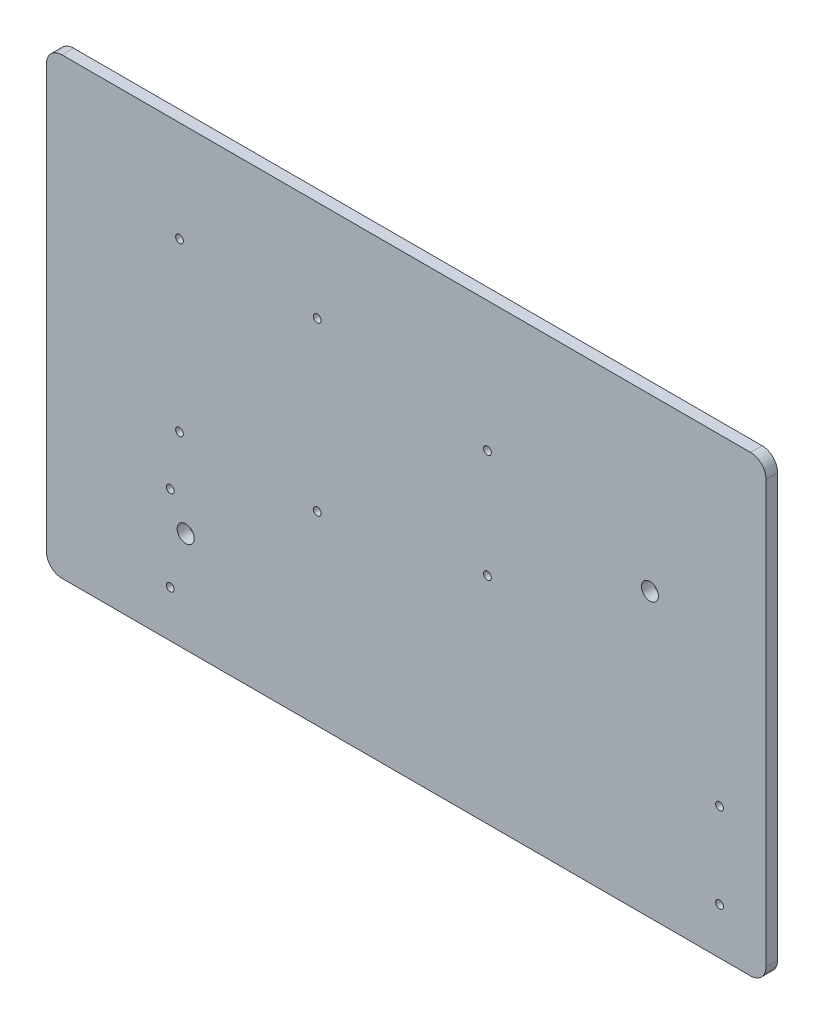
SolidWorks part; units mm, degrees
ref_plane "Front Plane" through (0, 0, 0) normal (0, 0, 1) x (1, 0, 0)
ref_plane "Top Plane" through (0, 0, 0) normal (0, 1, 0) x (1, 0, 0)
ref_plane "Right Plane" through (0, 0, 0) normal (1, 0, 0) x (0, 0, -1)
sketch "Sketch 1" plane through (0, 0, 0) normal (0, 0, 1) x (1, 0, 0)
  line L0 (0, 551.1662) -> (0, -654.445) construction
  line L1 (65, 78.3543) -> (65, -162.0992) construction
  line L2 (-115, -209.4546) -> (-115, 263.3834) construction
  line L3 (-293, 55) -> (383.7528, 55) construction
  line L4 (-115, 163) -> (-440.2764, 163) construction
  line L5 (-465, -273) -> (-465, 273)
  line L6 (-445, 293) -> (445, 293)
  line L7 (-92.1776, 0) -> (566.073, 0) construction
  line L8 (-308.5808, -178) -> (40.9999, -178) construction
  line L9 (-325, -103) -> (425, -103) construction
  line L10 (-325, -103) -> (-325, -253) construction
  line L11 (-293, 163) -> (-293, -53) construction
  line L12 (-455, 198.6727) -> (-455, -162.0992) construction
  line L13 (425, -103) -> (425, -253) construction
  line L14 (-445, -293) -> (445, -293)
  line L15 (465, -273) -> (465, 273)
  line L16 (425, -253) -> (-325, -253) construction
  line L17 (50, -103) -> (50, -253) construction
  line L18 (315, 72.5) -> (315, 2.5) construction
  circle A0 centre (-115, 163) radius 5
  circle A2 centre (-293, 163) radius 5
  circle A3 centre (-293, -53) radius 5
  circle A4 centre (105, -15) radius 5
  circle A6 centre (-115, -53) radius 5
  circle A7 centre (105, 125) radius 5
  circle A8 centre (-305, -123) radius 5
  circle A9 centre (-305, -233) radius 5
  circle A12 centre (405, -233) radius 5
  circle A13 centre (405, -123) radius 5
  circle A14 centre (315, 72.5) radius 11
  circle A15 centre (315, 2.5) radius 11 construction
  circle A16 centre (-285, -163) radius 11
  arc A17 (-445, -293) -> (-465, -273) centre (-445, -273) cw
  arc A18 (465, -273) -> (445, -293) centre (445, -273) cw
  arc A19 (465, 273) -> (445, 293) centre (445, 273) ccw
  arc A20 (-465, 273) -> (-445, 293) centre (-445, 273) cw
  point P34 (-585, 0)
  point P38 (-325, -178)
  point P44 (-465, 0)
  point P46 (0, -293)
  point P47 (0, 293)
  point P49 (0, -253)
  point P52 (0, -103)
  point P61 (-465, -293)
  point P64 (465, -293)
  point P67 (465, 293)
  point P70 (-465, 293)
  dimension "D1" = 10
  dimension "D2" = 216
  dimension "D3" = 178
  dimension "D4" = 10
  dimension "D5" = 140
  dimension "D6" = 220
  dimension "D8" = 400
  dimension "D16" = 586
  dimension "D17" = 130
  dimension "D18" = 40
  dimension "D9" = 10
  dimension "D12" = 75
  dimension "D14" = 20
  dimension "D15" = 750
  dimension "D20" = 22
  dimension "D21" = 150
  dimension "D22" = 35
  dimension "D24" = 22
  dimension "D25" = 40
  dimension "D26" = 20
  dimension "D27" = 15
  dimension "D7" = 40
  dimension "D10" = 162
  dimension "D11" = 10
  dimension "D13" = 20
  dimension "D19" = 50
  dimension "D23" = 70
extrude "Boss-Extrude 1" add sketch "Sketch 1" along normal blind 15
